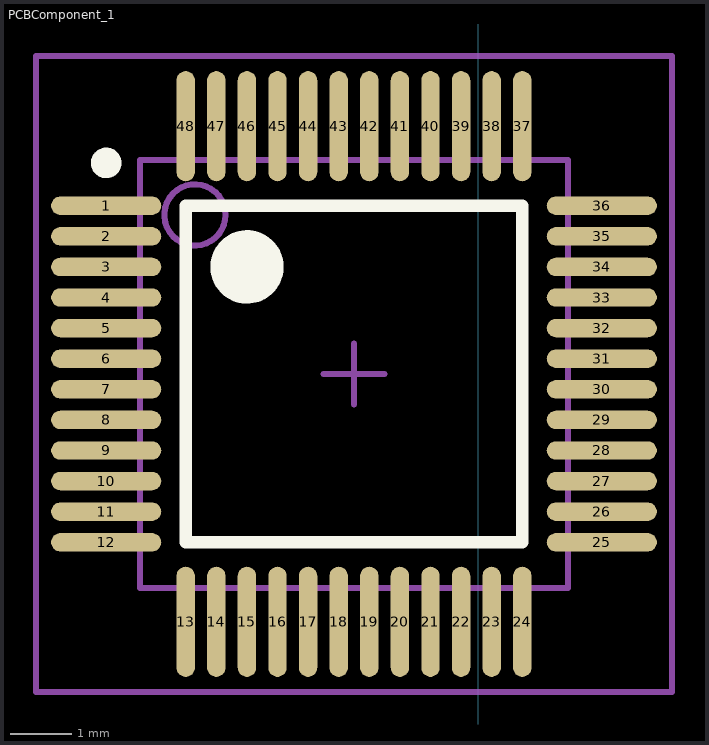
[diagram p0: the footprint, top view; thin cyan lines are the x and y axes]
# Altium footprint library MISC80722-6.PcbLib: 1 footprints
Each footprint in its own frame and in the unit in brackets; x right, y up, seen from the top. Pads: shape width x height; smd on the part's side, far side on the other; paste and mask are expansions set on the pad; w line width, h text height; cw(c..) or ccw(c..) is an arc to the next point about the centre after c.

## PCBComponent_1 [mm]
pads (48):
  oval 1.8x0.3 smd: 1(-6.082,-4.362) 2(-6.082,-4.862) 3(-6.082,-5.362) 4(-6.082,-5.862) 5(-6.082,-6.362) 6(-6.082,-6.862) 7(-6.082,-7.362) 8(-6.082,-7.862) 9(-6.082,-8.362) 10(-6.082,-8.862) 11(-6.082,-9.362) 12(-6.082,-9.862) 25(2.018,-9.862) 26(2.018,-9.362) 27(2.018,-8.862) 28(2.018,-8.362) 29(2.018,-7.862) 30(2.018,-7.362) 31(2.018,-6.862) 32(2.018,-6.362) 33(2.018,-5.862) 34(2.018,-5.362) 35(2.018,-4.862) 36(2.018,-4.362)
  oval 0.3x1.8 smd: 13(-4.782,-11.162) 14(-4.282,-11.162) 15(-3.782,-11.162) 16(-3.282,-11.162) 17(-2.782,-11.162) 18(-2.282,-11.162) 19(-1.782,-11.162) 20(-1.282,-11.162) 21(-0.782,-11.162) 22(-0.282,-11.162) 23(0.218,-11.162) 24(0.718,-11.162) 37(0.718,-3.062) 38(0.218,-3.062) 39(-0.282,-3.062) 40(-0.782,-3.062) 41(-1.282,-3.062) 42(-1.782,-3.062) 43(-2.282,-3.062) 44(-2.782,-3.062) 45(-3.282,-3.062) 46(-3.782,-3.062) 47(-4.282,-3.062) 48(-4.782,-3.062)
Top Overlay:
  circle w0.25: c-6.082,-3.662 r0.125
  circle w0.6: c-3.782,-5.362 r0.3
  lines w0.2: -4.782,-9.862 -4.782,-4.362 0.718,-4.362 0.718,-9.862 -4.782,-9.862
Mechanical 13:
  circle w0.1: c-4.632,-4.512 r0.5
  lines w0.1: -5.532,-10.612 -5.532,-3.612 1.468,-3.612 1.468,-10.612 -5.532,-10.612
Mechanical 15:
  lines w0.1: -2.532,-7.112 -1.532,-7.112 ; -2.032,-7.612 -2.032,-6.612 ; -7.232,-12.312 -7.232,-1.912 3.168,-1.912 3.168,-12.312 -7.232,-12.312
3D body: height 1.6, standoff 0, extent -5.532,-10.612 1.468,-3.612